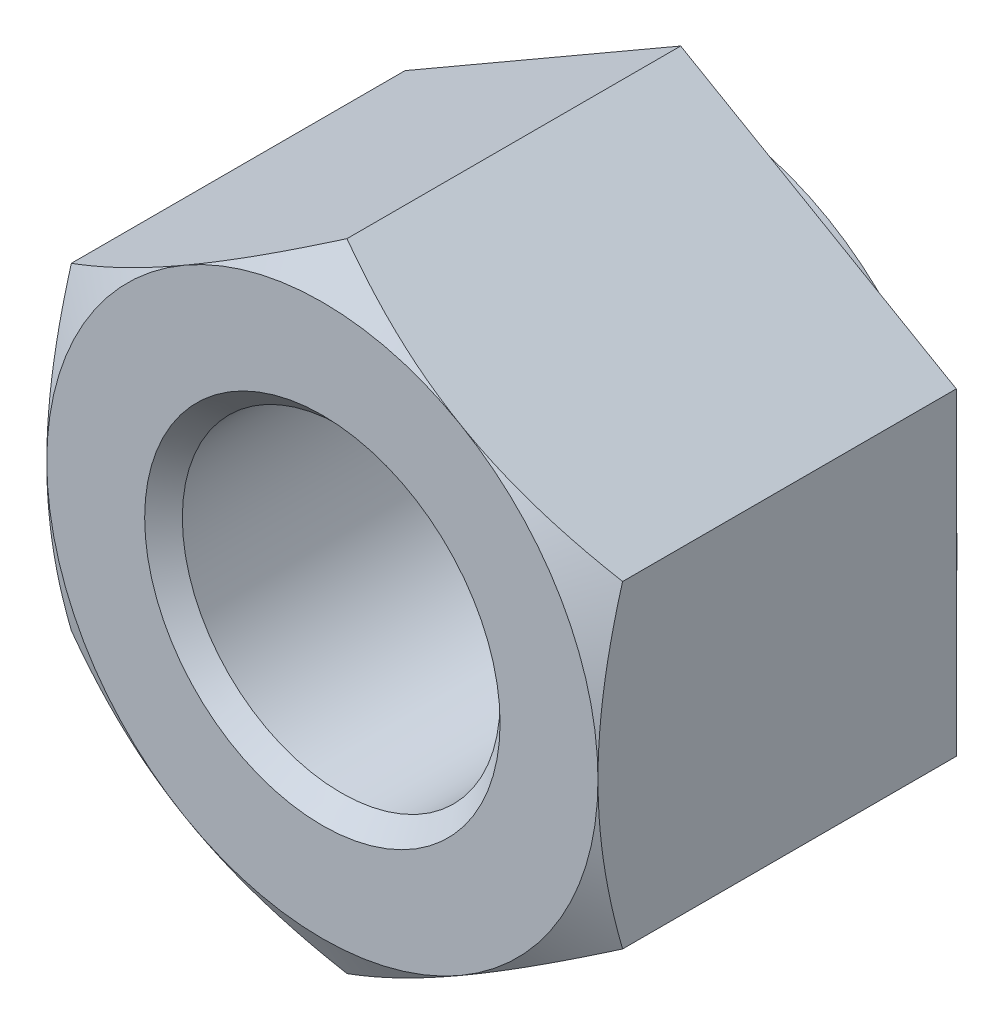
from build123d import *

# Parameters (mm, degrees)
SKETCH1_R          = 6.9175
EXTRUDE1_DEPTH     = 16.4
SKETCH2_OUTSIDE_W  = 34.032
SKETCH2_OUTSIDE_H  = 37.744
SKETCH2_OUTSIDE_R  = 11.25
CUT_EXTRUDE2_DEPTH = 0.8
SKETCH3_OUTSIDE_W  = 122.7
SKETCH3_OUTSIDE_H  = 126.412
SKETCH3_OUTSIDE_R  = 12
CUT_EXTRUDE3_DEPTH = 25.595934623
CUT_EXTRUDE3_DRAFT = -60
CHAMFER1_SIZE      = 0.82


with BuildPart() as part:
    # Sketch1 → Extrude1 (new body)
    with BuildSketch(Plane.XY):
        Polygon((0, 13.856406461), (-12, 6.92820323), (-12, -6.92820323), (0, -13.856406461), (12, -6.92820323), (12, 6.92820323), align=None)
        Circle(SKETCH1_R, mode=Mode.SUBTRACT)
    extrude(amount=EXTRUDE1_DEPTH)

    # Sketch2 outside → Cut-Extrude2 (cut)
    with BuildSketch(Plane.XY):
        Rectangle(SKETCH2_OUTSIDE_W, SKETCH2_OUTSIDE_H)
        Circle(SKETCH2_OUTSIDE_R, mode=Mode.SUBTRACT)
    extrude(amount=CUT_EXTRUDE2_DEPTH, mode=Mode.SUBTRACT)


with BuildPart() as cut_extrude3_tool:
    # Sketch3 outside → Cut-Extrude3 (with draft: the straight prism first)
    with BuildSketch(Plane.XY.offset(16.4)):
        Rectangle(SKETCH3_OUTSIDE_W, SKETCH3_OUTSIDE_H)
        Circle(SKETCH3_OUTSIDE_R, mode=Mode.SUBTRACT)
    extrude(amount=-CUT_EXTRUDE3_DEPTH)
    # Cut-Extrude3: the draft: its side faces are tilted about the plane it starts from
    cut_extrude3_sides = [cut_extrude3_tool.faces().sort_by_distance(p)[0] for p in [
        (0, -63.206, 3.602032688),
        (61.35, 0, 3.602032688),
        (0, 63.206, 3.602032688),
        (-61.35, 0, 3.602032688),
        (-12, 0, 3.602032688),
    ]]
    draft(cut_extrude3_sides, Plane.XY.offset(16.4), CUT_EXTRUDE3_DRAFT)


with BuildPart() as part_1:
    add(part.part)

    # Cut-Extrude3: cut by cut_extrude3_tool
    add(cut_extrude3_tool.part, mode=Mode.SUBTRACT)

    # Chamfer1
    chamfer1_edges = [part_1.edges().sort_by_distance(p)[0] for p in [
        (-6.9175, 0, 0),
        (-6.9175, 0, 16.4),
    ]]
    chamfer(chamfer1_edges, length=CHAMFER1_SIZE)


solid = part_1.part
